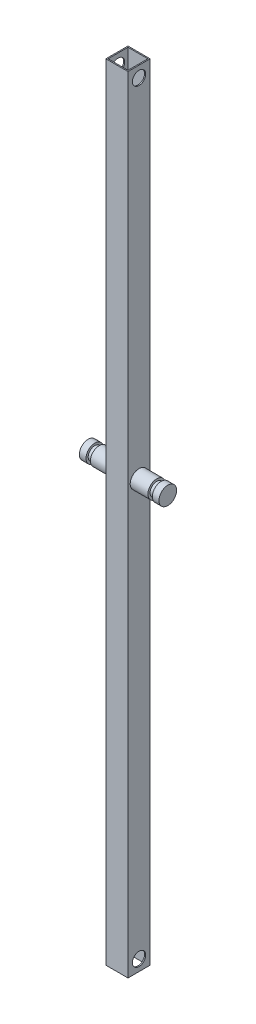
SolidWorks part; units mm, degrees
ref_plane "Front Plane" through (0, 0, 0) normal (0, 0, 1) x (1, 0, 0)
ref_plane "Top Plane" through (0, 0, 0) normal (0, 1, 0) x (1, 0, 0)
ref_plane "Right Plane" through (0, 0, 0) normal (1, 0, 0) x (0, 0, -1)
sketch "Sketch1" plane through (0, 0, 0) normal (0, 1, 0) x (1, 0, 0)
  line L0 (4.5, 4.5) -> (4.5, -4.5)
  line L1 (-5, 5) -> (5, 5)
  line L2 (-5, 5) -> (-5, -5)
  line L3 (-5, -5) -> (5, -5)
  line L4 (5, 5) -> (5, -5)
  line L5 (-5, 5) -> (5, -5) construction
  line L6 (-5, -5) -> (5, 5) construction
  line L7 (-4.5, -4.5) -> (4.5, -4.5)
  line L8 (-4.5, 4.5) -> (-4.5, -4.5)
  line L9 (-4.5, 4.5) -> (4.5, 4.5)
  point P0 (0, 0)
  dimension "D1" = 10
  dimension "D2" = 0.5
extrude "Boss-Extrude1" add sketch "Sketch1" along normal blind 355
sketch "Sketch2" plane through (5, 0, 0) normal (1, 0, 0) x (0, 0, -1)
  line L0 (-5, 0) -> (5, 0) construction
  line L1 (5, 355) -> (5, 0) construction
  circle A0 centre (0, 193) radius 4
  dimension "D1" = 8
  dimension "D2" = 193
  dimension "D3" = 5
extrude "Boss-Extrude2" add sketch "Sketch2" along normal blind 8
sketch "Sketch3" plane through (13, 0, 0) normal (1, 0, 0) x (0, 0, -1)
  circle A0 centre (0, 193) radius 3
  dimension "D1" = 6
extrude "Boss-Extrude3" add sketch "Sketch3" along normal blind 2
sketch "Sketch4" plane through (15, 0, 0) normal (1, 0, 0) x (0, 0, -1)
  circle A0 centre (0, 193) radius 4
extrude "Boss-Extrude4" add sketch "Sketch4" along normal blind 3
mirror "Mirror1" about plane through (0, 0, 0) normal (1, 0, 0) of bodies 109
sketch "Sketch5" plane through (5, 0, 0) normal (1, 0, 0) x (0, 0, -1)
  line L0 (5, 355) -> (5, 0) construction
  circle A0 centre (0, 5) radius 3
  dimension "D1" = 6
  dimension "D2" = 5
  dimension "D3" = 5
extrude "Cut-Extrude1" cut sketch "Sketch5" against normal blind 21
sketch "Sketch6" plane through (-5, 0, 0) normal (-1, 0, 0) x (0, 0, 1)
  line L0 (-5, 355) -> (5, 355) construction
  line L1 (5, 355) -> (5, 0) construction
  circle A0 centre (0, 350) radius 3
  dimension "D1" = 6
  dimension "D2" = 5
  dimension "D3" = 5
extrude "Cut-Extrude2" cut sketch "Sketch6" against normal blind 18
